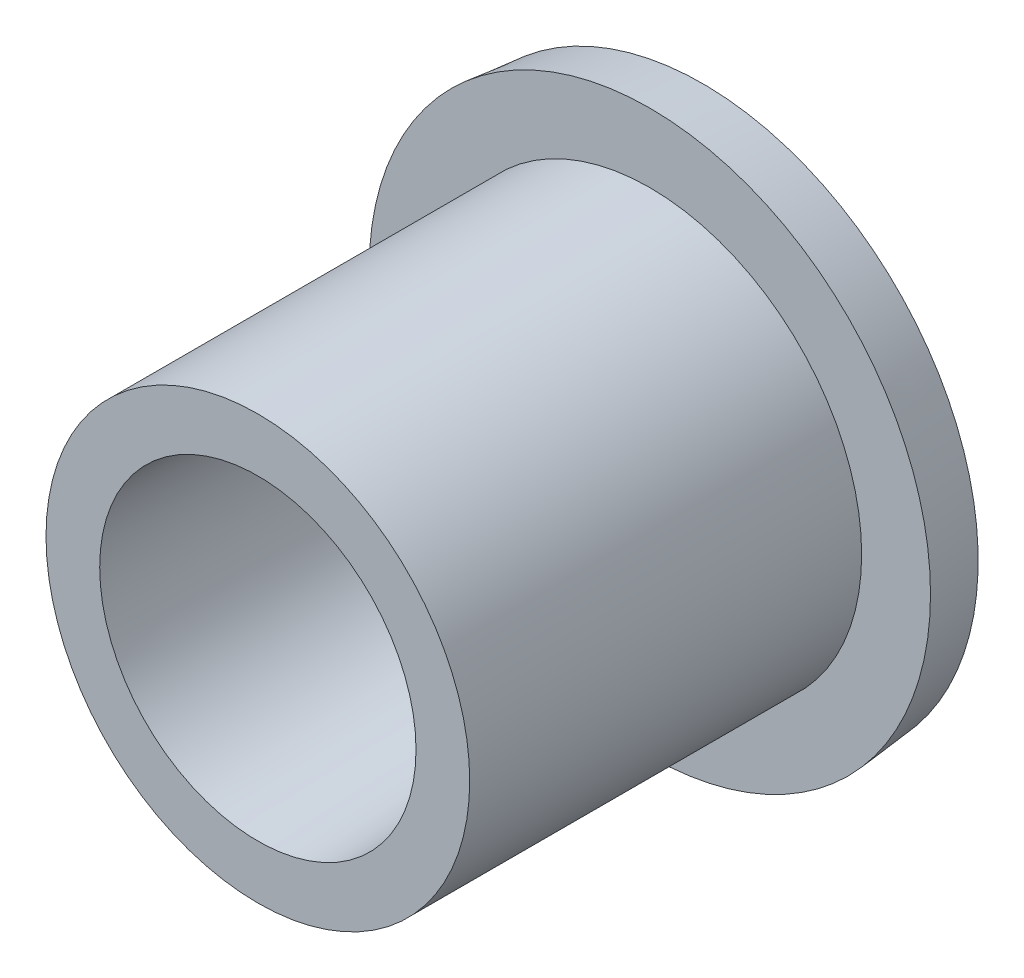
from build123d import *


with BuildPart() as part:
    # Sketch1 → Revolve1 (revolve)
    with BuildSketch(Plane(origin=(0, 318.5, 0), x_dir=(-1, 0, 0), z_dir=(0, -1, 0))):
        Polygon((40, 164.5), (40, 90.5), (29.862068966, 90.5), (26, 174.5), (52, 174.5), (53, 164.5), align=None)
    revolve(axis=Axis((0, 318.5, -174.5), (0, 0, 1)))


solid = part.part
